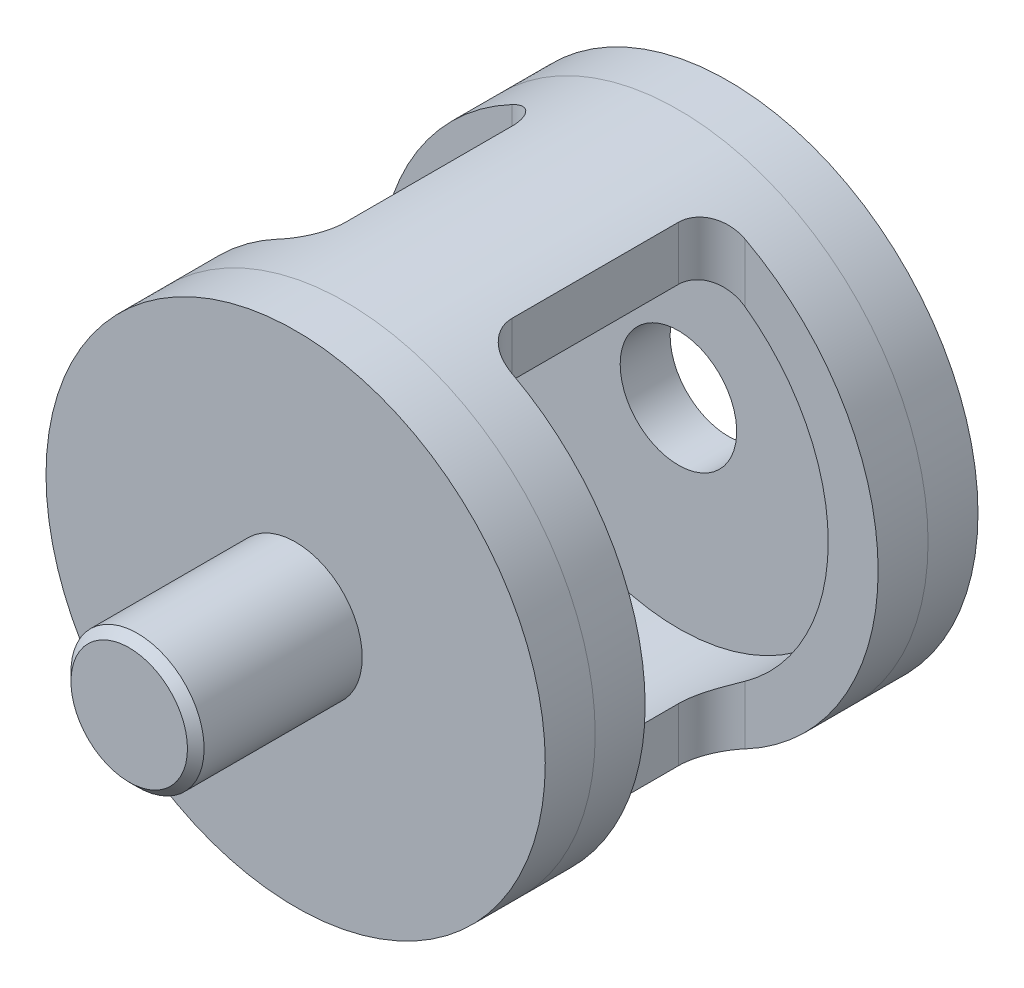
SolidWorks part; units mm, degrees
material "Q235"
ref_plane "Front Plane" through (0, 0, 0) normal (0, 0, 1) x (1, 0, 0)
ref_plane "Top Plane" through (0, 0, 0) normal (0, 1, 0) x (1, 0, 0)
ref_plane "Right Plane" through (0, 0, 0) normal (1, 0, 0) x (0, 0, -1)
sketch "Sketch1" plane through (0, 0, 0) normal (0, 0, 1) x (1, 0, 0)
  circle A0 centre (0, 0) radius 15
  circle A1 centre (0, 0) radius 12
  dimension "D1" = 30
  dimension "D2" = 3
extrude "Boss-Extrude1" add sketch "Sketch1" along normal blind 20
sketch "Sketch2" plane through (0, 0, 0) normal (0, 1, 0) x (1, 0, 0)
  line L0 (-15, 0) -> (-15, -20) construction
  line L5 (-15, -3) -> (-5, -3)
  line L6 (-15, -3) -> (-15, -17)
  line L7 (-15, -17) -> (-5, -17)
  line L8 (-5, -3) -> (-5, -17)
  line L9 (0, 0) -> (0, -20) construction
  line L10 (12, 0) -> (-12, 0) construction
  line L11 (-15, -20) -> (15, -20) construction
  line L12 (5, -3) -> (5, -17)
  line L13 (15, -17) -> (5, -17)
  line L14 (15, -3) -> (15, -17)
  line L15 (15, -3) -> (5, -3)
extrude "Cut-Extrude1" cut sketch "Sketch2" against normal through all both and the other way through all
sketch "Sketch3" plane through (0, 0, 20) normal (0, 0, 1) x (1, 0, 0)
  circle A1 centre (0, 0) radius 15
  circle A2 centre (0, 0) radius 15
  dimension "D1" = 0
extrude "Boss-Extrude2" add sketch "Sketch3" along normal blind 3 separate body
sketch "Sketch5" plane through (0, 0, 0) normal (0, 0, -1) x (-1, 0, 0)
  circle A1 centre (0, 0) radius 15
  circle A2 centre (0, 0) radius 15
  dimension "D1" = 0
extrude "Boss-Extrude3" add sketch "Sketch5" along normal blind 3 separate body
hole_wizard "M6 Clearance Hole1" positions "Sketch6" profile "Sketch8" hole size "M6" standard "GB"
sketch "Sketch6" plane through (0, 0, -3) normal (0, 0, -1) x (-1, 0, 0)
  point P0 (0, 0)
sketch "Sketch8" plane through (0, 0, -3) normal (1, 0, 0) x (0, 1, 0)
  line L0 (0, 0) -> (0, 7.103)
  line L1 (0, 7.103) -> (3.5, 5)
  line L2 (3.5, 5) -> (3.5, 0)
  line L5 (3.5, 0) -> (0, 0)
  line L10 (0, 7.103) -> (-3.5, 5) construction
  line L11 (0, -6.35) -> (0, 107.95) construction
  dimension "孔直径" = 7
  dimension "孔深度" = 5
  dimension "导头角度" = 118
hole_wizard "M8 Tapped Hole1" positions "Sketch9" profile "Sketch10" tap size "M8" standard "GB"
sketch "Sketch9" plane through (0, 0, 23) normal (0, 0, 1) x (1, 0, 0)
  point P0 (0, 0)
sketch "Sketch10" plane through (0, 0, 23) normal (1, 0, 0) x (0, -1, 0)
  line L0 (0, 0) -> (0, 12.0429)
  line L1 (0, 12.0429) -> (3.4, 10)
  line L2 (3.4, 10) -> (3.4, 0)
  line L5 (3.4, 0) -> (0, 0)
  line L10 (0, 12.0429) -> (-3.4, 10) construction
  line L11 (0, -6.35) -> (0, 107.95) construction
  dimension "螺纹孔钻头直径" = 6.8
  dimension "螺纹孔钻头深度" = 10
  dimension "导头角度" = 118
cosmetic thread "Cosmetic thread1" parameters "D1"=3, "D2"=8
sketch "Sketch11" plane through (0, 0, 23) normal (0, 0, 1) x (1, 0, 0)
  circle A0 centre (0, 0) radius 4
  dimension "D1" = 8
extrude "Boss-Extrude4" add sketch "Sketch11" along normal blind 10
fillet "Fillet1" radius 2 8 edges at (-5, -12.5254, 3) (-5, 12.5254, 3) (-5, 12.5254, 17) (-5, -12.5254, 17) (5, 12.5254, 3) (5, -12.5254, 3) (5, -12.5254, 17) (5, 12.5254, 17)
chamfer "Chamfer1" distance 0.5 angle 45 1 edges at (4, 0, 33)
equation "\"D3@Sketch2\"=\"D2@Sketch2\""
